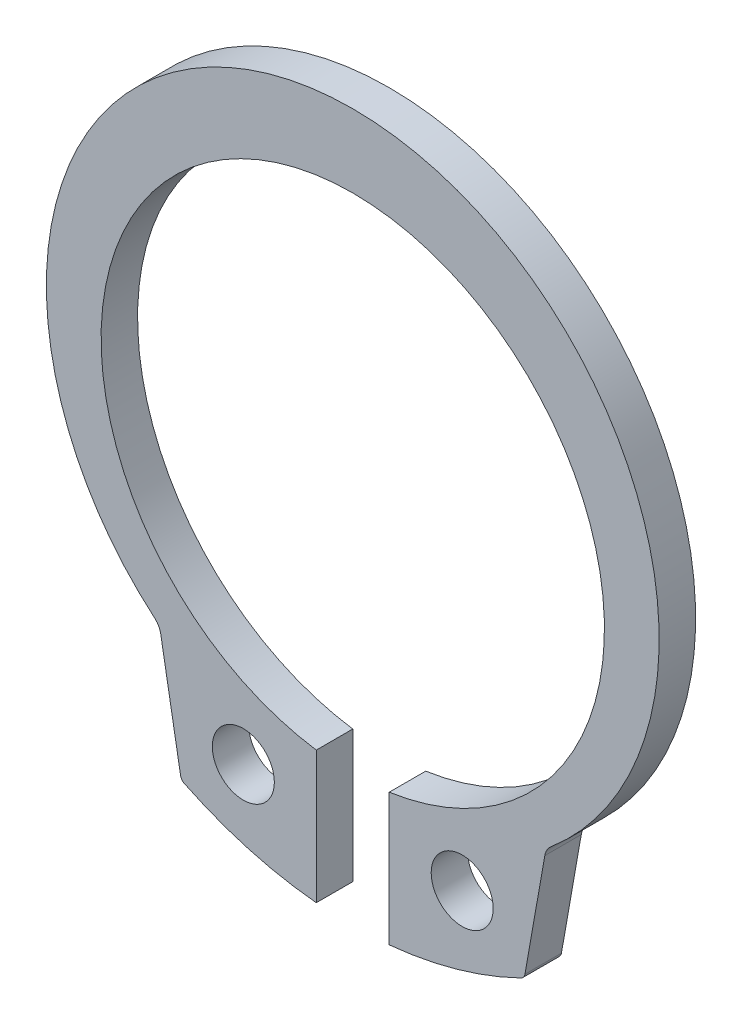
SolidWorks part; units mm, degrees
ref_plane "Front" through (0, 0, 0) normal (0, 0, 1) x (1, 0, 0)
ref_plane "Top" through (0, 0, 0) normal (0, 1, 0) x (1, 0, 0)
ref_plane "Right" through (0, 0, 0) normal (1, 0, 0) x (0, 0, -1)
sketch "Sketch1" plane through (0, 0, 0) normal (0, 0, 1) x (1, 0, 0)
  line L0 (0, 4.2365) -> (0, -4.9012) construction
  line L1 (-1, -7.3272) -> (-1, -10.9523)
  line L2 (1, -7.3272) -> (1, -10.9523)
  line L3 (8.7, -0.5) -> (-8.7, -0.5) construction
  line L4 (5.297, -6.5194) -> (4.703, -9.8878)
  line L7 (-5.297, -6.5194) -> (-4.703, -9.8878)
  line L8 (-5.297, -6.5194) -> (-5.297, -14.5901) construction
  arc A0 (1, -7.3272) -> (-1, -7.3272) centre (0, -0.5) ccw
  arc A1 (5.297, -6.5194) -> (-5.297, -6.5194) centre (0, 0) ccw
  arc A2 (-8.7, -0.5) -> (8.7, -0.5) centre (0, -0.5) ccw construction
  arc A3 (4.703, -9.8878) -> (1, -10.9523) centre (0, -0.5) cw
  arc A4 (-4.703, -9.8878) -> (-1, -10.9523) centre (0, -0.5) ccw
  circle A5 centre (3, -8.6664) radius 0.85
  circle A6 centre (-3, -8.6664) radius 0.85
  point P17 (-5, -8.2036)
  dimension "d" = 13.8
  dimension "D2" = 10
  dimension "d0" = 16.8
  dimension "d1" = 1.7
  dimension "R1" = 8.7
  dimension "R" = 10.5
  dimension "B1" = 2
  dimension "C" = 0.5
  dimension "L" = 10
  dimension "B2" = 6
extrude "Body" add sketch "Sketch1" against normal blind 1
fillet "Fillet1" radius 0.2 2 edges at (-4.703, -9.8878, -0.5) (4.703, -9.8878, -0.5)
fillet "Fillet2" radius 0.5 2 edges at (5.297, -6.5194, -0.5) (-5.297, -6.5194, -0.5)
